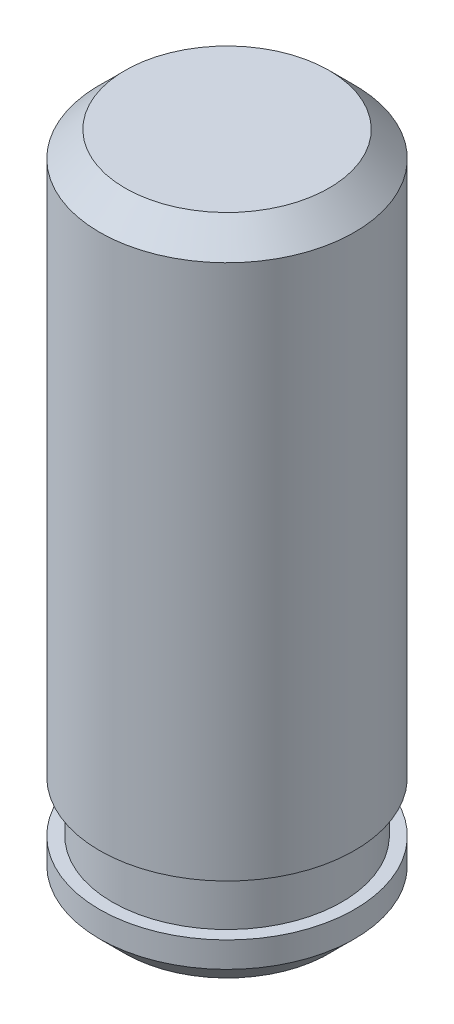
SolidWorks part; units mm, degrees
ref_plane "Front Plane" through (0, 0, 0) normal (0, 0, 1) x (1, 0, 0)
ref_plane "Top Plane" through (0, 0, 0) normal (0, 1, 0) x (1, 0, 0)
ref_plane "Right Plane" through (0, 0, 0) normal (1, 0, 0) x (0, 0, -1)
other "Configuration Table"
sketch "Sketch1" plane through (0, 0, 0) normal (0, 1, 0) x (1, 0, 0)
  circle A0 centre (0, 0) radius 2.5
  dimension "D1" = 5
extrude "Boss-Extrude1" add sketch "Sketch1" along normal blind 1
sketch "Sketch2" plane through (0, 1, 0) normal (0, 1, 0) x (1, 0, 0)
  circle A0 centre (0, 0) radius 2.25
  dimension "D1" = 4.5
extrude "Boss-Extrude2" add sketch "Sketch2" along normal blind 1
sketch "Sketch3" plane through (0, 2, 0) normal (0, 1, 0) x (1, 0, 0)
  circle A0 centre (0, 0) radius 2.5
  dimension "D1" = 5
extrude "Boss-Extrude3" add sketch "Sketch3" along normal blind 11
chamfer "Chamfer1" distance 0.5 angle 45 2 edges at (0, 0, 2.5) (0, 13, 2.5)
